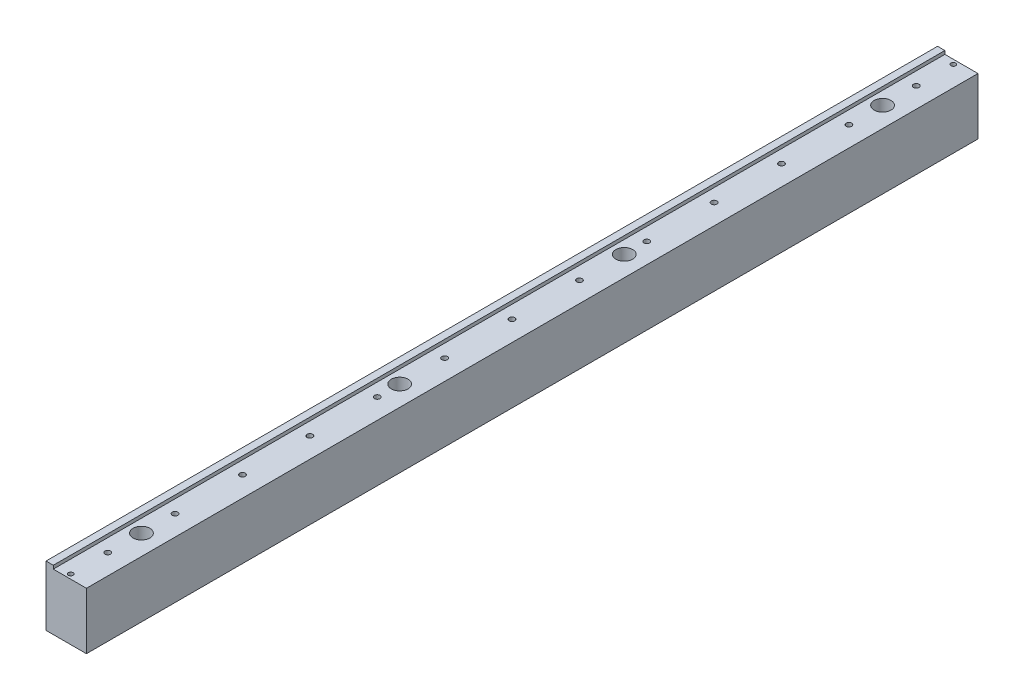
from build123d import *

# Parameters (mm, degrees)
EXTRUDE_1_DEPTH           = 397
HOLE_WIZARD_M6_1_D        = 5
HOLE_WIZARD_M6_1_DEPTH    = 15
HOLE_WIZARD_M6_1_TIP      = 1.502151548
PATTERN_LINEAR_1_COUNT    = 13
PATTERN_LINEAR_1_PITCH    = 60
HOLE_WIZARD_1_D           = 9
HOLE_WIZARD_1_CBORE_D     = 15
HOLE_WIZARD_1_CBORE_DEPTH = 15
HOLE_WIZARD_M5_1_D        = 4.2
HOLE_WIZARD_M5_1_DEPTH    = 12.4
HOLE_WIZARD_M5_1_TIP      = 1.2618073


with BuildPart() as part:
    # 草图1 → 凸台-拉伸1 (new, symmetric)
    with BuildSketch(Plane.XY):
        Polygon((0, 0), (36, 0), (36, 50.5), (6.5, 50.5), (6.5, 53.5), (0, 53.5), align=None)
    extrude(amount=EXTRUDE_1_DEPTH, both=True)

    # M6 螺纹孔1
    with Locations(Plane.ZY):
        with Locations((-320, 28.5), (270, 28.5)):
            Hole(HOLE_WIZARD_M6_1_D / 2, depth=HOLE_WIZARD_M6_1_DEPTH)
            with Locations((0, 0, -(HOLE_WIZARD_M6_1_DEPTH + HOLE_WIZARD_M6_1_TIP / 2))):  # 118° drill point
                Cone(0, HOLE_WIZARD_M6_1_D / 2, HOLE_WIZARD_M6_1_TIP, mode=Mode.SUBTRACT)

    # 草图4 → M6 螺纹孔2 (revolve, cut)
    with BuildSketch(Plane(origin=(18, 50.5, -360), x_dir=(0, 0, 1), z_dir=(1, 0, 0))):
        Polygon((0, 0), (0, 16.502151548), (2.5, 15), (2.5, 0), align=None)
    hole_wizard_m6_2 = revolve(axis=Axis((18, 56.85, -360), (0, -1, 0)), mode=Mode.SUBTRACT)

    # 阵列(线性)1: M6 螺纹孔2 ×13
    with Locations(*[(0, 0, i * PATTERN_LINEAR_1_PITCH) for i in range(1, PATTERN_LINEAR_1_COUNT)]):
        add(hole_wizard_m6_2, mode=Mode.SUBTRACT)

    # 打孔尺寸(%根据)内六角圆柱头螺钉的类型1 (through all)
    with Locations(Plane(origin=(0, 50.5, 0), x_dir=(1, 0, 0), z_dir=(0, 1, 0))):
        with Locations((18, 330), (18, 100), (18, -100), (18, -330)):
            CounterBoreHole(HOLE_WIZARD_1_D / 2, HOLE_WIZARD_1_CBORE_D / 2, HOLE_WIZARD_1_CBORE_DEPTH)

    # M5 螺纹孔1
    with Locations(Plane(origin=(0, 50.5, 0), x_dir=(1, 0, 0), z_dir=(0, 1, 0))):
        with Locations((18, 393), (18, -393)):
            Hole(HOLE_WIZARD_M5_1_D / 2, depth=HOLE_WIZARD_M5_1_DEPTH)
            with Locations((0, 0, -(HOLE_WIZARD_M5_1_DEPTH + HOLE_WIZARD_M5_1_TIP / 2))):  # 118° drill point
                Cone(0, HOLE_WIZARD_M5_1_D / 2, HOLE_WIZARD_M5_1_TIP, mode=Mode.SUBTRACT)


solid = part.part
